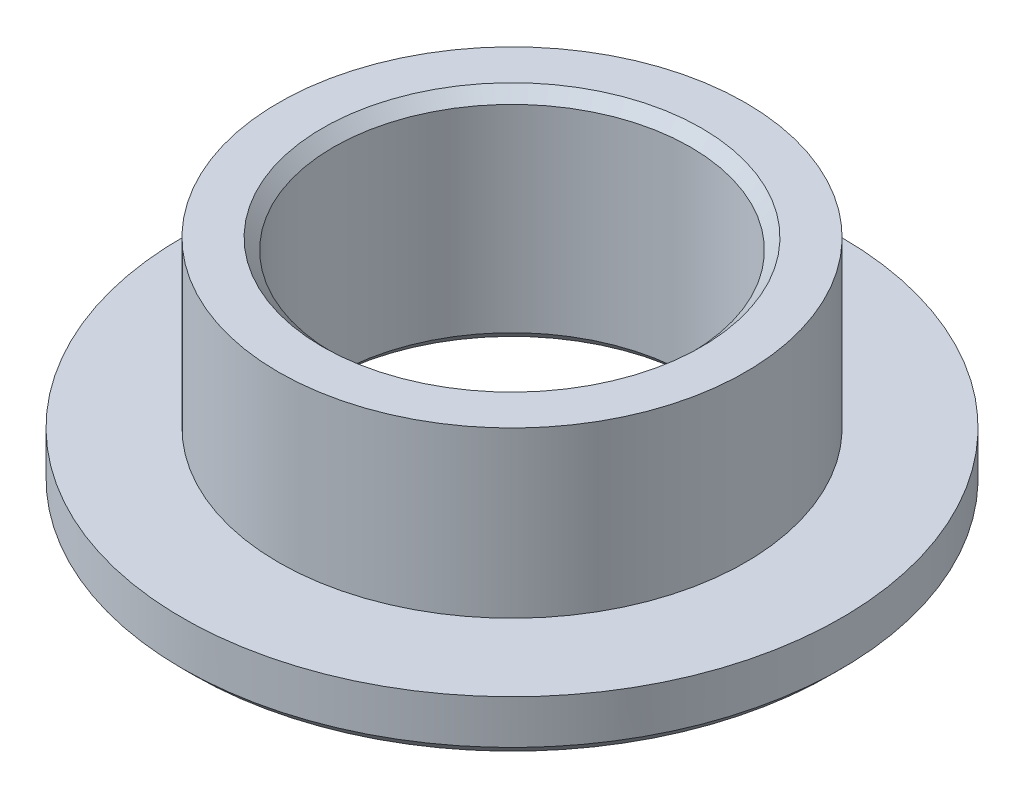
from build123d import *

# Parameters (mm, degrees)
CHAMFER1_SIZE = 2


with BuildPart() as part:
    # Sketch1 → Revolve1 (revolve)
    with BuildSketch(Plane.XY, mode=Mode.PRIVATE) as revolve1_sk:
        Polygon((-32.5, 0), (-32.5, 40), (-42.5, 40), (-42.5, 10), (-60, 10), (-60, 0), align=None)
    revolve(revolve1_sk.sketch.rotate(Axis((0, 0, 0), (0, 1, 0)), 270), axis=Axis((0, 0, 0), (0, 1, 0)))

    # Chamfer1
    chamfer1_edges = [part.edges().sort_by_distance(p)[0] for p in [
        (0, 0, 60),
        (0, 40, 32.5),
        (0, 0, 32.5),
    ]]
    chamfer(chamfer1_edges, length=CHAMFER1_SIZE)


solid = part.part
